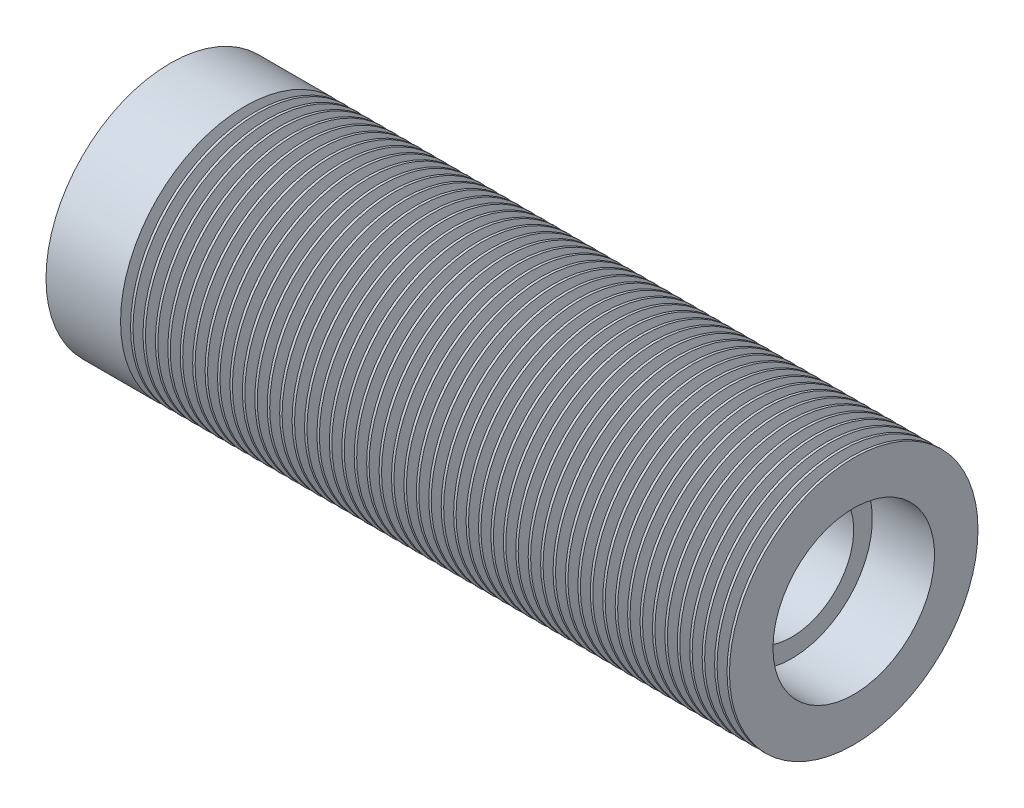
from build123d import *


with BuildPart() as part:
    # Sketch1 → Revolve1 (revolve)
    with BuildSketch(Plane.XY, mode=Mode.PRIVATE) as revolve1_sk:
        Polygon((0, 6.5), (0, 10), (6, 10), (6.401923789, 8.5), (6.803847577, 10), (7, 10), (7.401923789, 8.5), (7.803847577, 10), (8, 10), (8.401923789, 8.5), (8.803847577, 10), (9, 10), (9.401923789, 8.5), (9.803847577, 10), (10, 10), (10.401923789, 8.5), (10.803847577, 10), (11, 10), (11.401923789, 8.5), (11.803847577, 10), (12, 10), (12.401923789, 8.5), (12.803847577, 10), (13, 10), (13.401923789, 8.5), (13.803847577, 10), (14, 10), (14.401923789, 8.5), (14.803847577, 10), (15, 10), (15.401923789, 8.5), (15.803847577, 10), (16, 10), (16.401923789, 8.5), (16.803847577, 10), (17, 10), (17.401923789, 8.5), (17.803847577, 10), (18, 10), (18.401923789, 8.5), (18.803847577, 10), (19, 10), (19.401923789, 8.5), (19.803847577, 10), (20, 10), (20.401923789, 8.5), (20.803847577, 10), (21, 10), (21.401923789, 8.5), (21.803847577, 10), (22, 10), (22.401923789, 8.5), (22.803847577, 10), (23, 10), (23.401923789, 8.5), (23.803847577, 10), (24, 10), (24.401923789, 8.5), (24.803847577, 10), (25, 10), (25.401923789, 8.5), (25.803847577, 10), (26, 10), (26.401923789, 8.5), (26.803847577, 10), (27, 10), (27.401923789, 8.5), (27.803847577, 10), (28, 10), (28.401923789, 8.5), (28.803847577, 10), (29, 10), (29.401923789, 8.5), (29.803847577, 10), (30, 10), (30.401923789, 8.5), (30.803847577, 10), (31, 10), (31.401923789, 8.5), (31.803847577, 10), (32, 10), (32.401923789, 8.5), (32.803847577, 10), (33, 10), (33.401923789, 8.5), (33.803847577, 10), (34, 10), (34.401923789, 8.5), (34.803847577, 10), (35, 10), (35.401923789, 8.5), (35.803847577, 10), (36, 10), (36.401923789, 8.5), (36.803847577, 10), (37, 10), (37.401923789, 8.5), (37.803847577, 10), (38, 10), (38.401923789, 8.5), (38.803847577, 10), (39, 10), (39.401923789, 8.5), (39.803847577, 10), (40, 10), (40.401923789, 8.5), (40.803847577, 10), (41, 10), (41.401923789, 8.5), (41.803847577, 10), (42, 10), (42.401923789, 8.5), (42.803847577, 10), (43, 10), (43.401923789, 8.5), (43.803847577, 10), (44, 10), (44.401923789, 8.5), (44.803847577, 10), (45, 10), (45.401923789, 8.5), (45.803847577, 10), (46, 10), (46.401923789, 8.5), (46.803847577, 10), (47, 10), (47.401923789, 8.5), (47.803847577, 10), (48, 10), (48.401923789, 8.5), (48.803847577, 10), (49, 10), (49.401923789, 8.5), (49.803847577, 10), (50, 10), (50.401923789, 8.5), (50.803847577, 10), (51, 10), (51.401923789, 8.5), (51.803847577, 10), (52, 10), (52.401923789, 8.5), (52.803847577, 10), (53, 10), (53.401923789, 8.5), (53.803847577, 10), (54, 10), (54.401923789, 8.5), (54.803847577, 10), (55, 10), (55, 6.5), (50, 6.5), (50, 5), (5, 5), (5, 6.5), align=None)
    revolve(revolve1_sk.sketch.rotate(Axis((0, 0, 0), (1, 0, 0)), 90), axis=Axis((0, 0, 0), (1, 0, 0)))


solid = part.part
